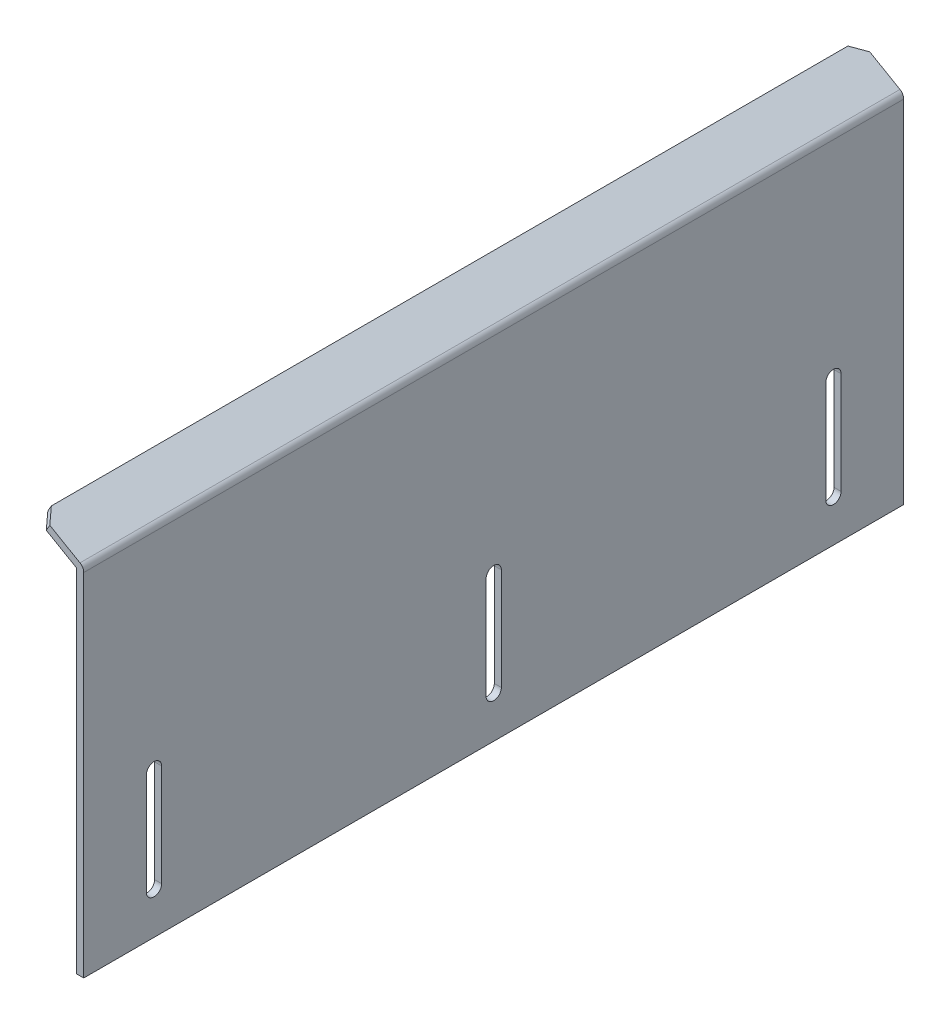
from build123d import *

# Parameters (mm, degrees)
EXTRUDE_1_DEPTH     = 350
CUT_EXTRUDE_1_DEPTH = 382.182371051
CUT_EXTRUDE_2_DEPTH = 382.182371051
CUT_EXTRUDE_3_DEPTH = 382.330464359
CHAMFER_1_SIZE      = 5
FILLET_1_R          = 0.2
FILLET_2_R          = 3.2


with BuildPart() as part:
    # 草图1 → 凸台-拉伸1 (new body)
    with BuildSketch(Plane.XY.offset(350)):
        Polygon((3, -150), (3, 1.732050808), (-15.820508076, 12.598076211), (-17.320508076, 10), (0, 0), (0, -150), align=None)
    extrude(amount=-EXTRUDE_1_DEPTH)

    # 草图2 → 切除-拉伸1 (cut, through all)
    with BuildSketch(Plane.ZY):
        with BuildLine():
            Line((316.75, -88.25), (316.75, -131.75))
            ThreePointArc((316.75, -131.75), (320, -135), (323.25, -131.75))
            Line((323.25, -131.75), (323.25, -88.25))
            ThreePointArc((323.25, -88.25), (320, -85), (316.75, -88.25))
        make_face()
    extrude(amount=-CUT_EXTRUDE_1_DEPTH, mode=Mode.SUBTRACT)

    # 草图3 → 切除-拉伸2 (cut, through all)
    with BuildSketch(Plane.ZY):
        with BuildLine():
            Line((26.75, -88.25), (26.75, -131.75))
            ThreePointArc((26.75, -131.75), (30, -135), (33.25, -131.75))
            Line((33.25, -131.75), (33.25, -88.25))
            ThreePointArc((33.25, -88.25), (30, -85), (26.75, -88.25))
        make_face()
    extrude(amount=-CUT_EXTRUDE_2_DEPTH, mode=Mode.SUBTRACT)

    # 草图4 → 切除-拉伸3 (cut, through all)
    with BuildSketch(Plane(origin=(3, 0, 0), x_dir=(0, 0, -1), z_dir=(1, 0, 0))):
        with BuildLine():
            Line((-171.75, -131.75), (-171.75, -88.25))
            ThreePointArc((-171.75, -88.25), (-175, -85), (-178.25, -88.25))
            Line((-178.25, -88.25), (-178.25, -131.75))
            ThreePointArc((-178.25, -131.75), (-175, -135), (-171.75, -131.75))
        make_face()
    extrude(amount=-CUT_EXTRUDE_3_DEPTH, mode=Mode.SUBTRACT)

    # 倒角1
    chamfer_1_edges = [part.edges().sort_by_distance(p)[0] for p in [
        (-16.570508076, 11.299038106, 0),
        (-16.570508076, 11.299038106, 350),
    ]]
    chamfer(chamfer_1_edges, length=CHAMFER_1_SIZE)

    # 圆角1
    fillet_1_edges = [part.edges().sort_by_distance(p)[0] for p in [
        (0, 0, 175),
    ]]
    fillet(fillet_1_edges, radius=FILLET_1_R)

    # 圆角2
    fillet_2_edges = [part.edges().sort_by_distance(p)[0] for p in [
        (3, 1.732050808, 175),
    ]]
    fillet(fillet_2_edges, radius=FILLET_2_R)


solid = part.part
